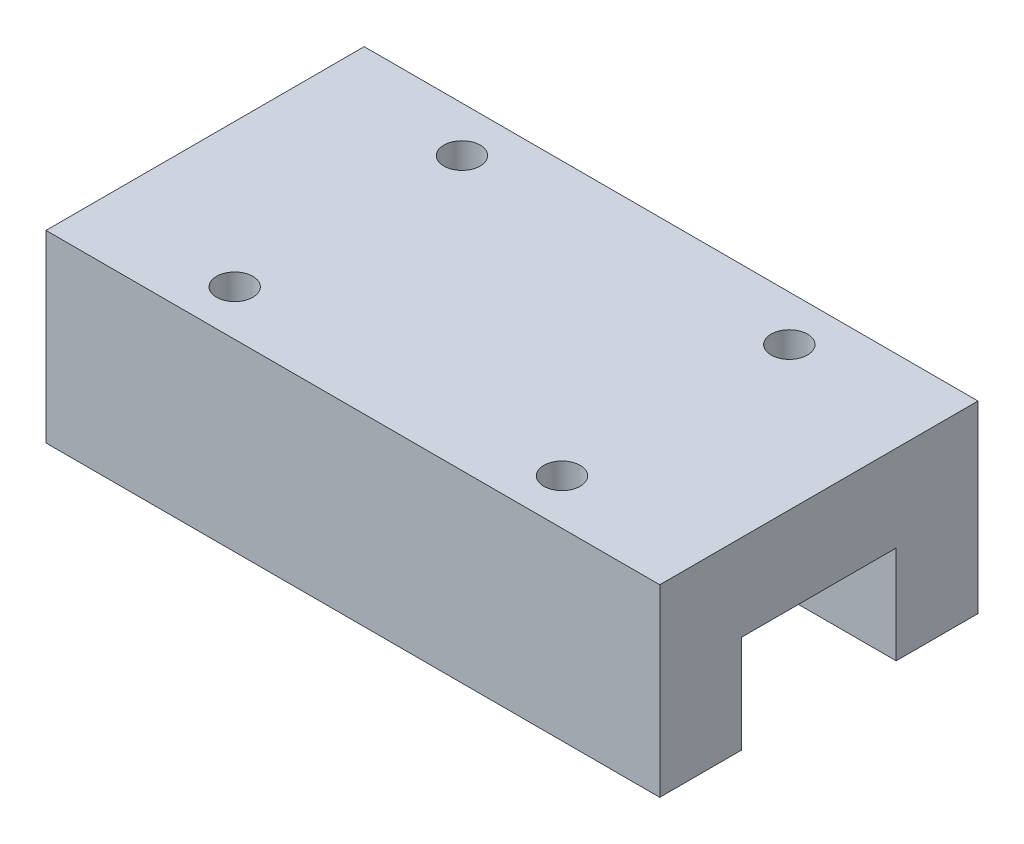
SolidWorks part; units mm, degrees
ref_plane "前视基准面" through (0, 0, 0) normal (0, 0, 1) x (1, 0, 0)
ref_plane "上视基准面" through (0, 0, 0) normal (0, 1, 0) x (1, 0, 0)
ref_plane "右视基准面" through (0, 0, 0) normal (1, 0, 0) x (0, 0, -1)
sketch "草图1" plane through (0, 0, 0) normal (0, 1, 0) x (1, 0, 0)
  line L1 (0, 0) -> (135, 0)
  line L2 (0, 0) -> (0, 70)
  line L3 (0, 70) -> (135, 70)
  line L4 (135, 0) -> (135, 70)
  dimension "D1" = 135
  dimension "D2" = 70
extrude "拉伸1" add sketch "草图1" along normal blind 40.5
sketch "草图2" plane through (0, 0, 0) normal (0, -1, 0) x (1, 0, 0)
  line L0 (135, 0) -> (135, -70) construction
  line L1 (135, -18) -> (0, -18)
  line L2 (135, -18) -> (135, -52)
  line L3 (135, -52) -> (0, -52)
  line L4 (0, -18) -> (0, -52)
  line L5 (0, -70) -> (0, 0) construction
  dimension "D1" = 34
  dimension "D2" = 18
extrude "切除-拉伸1" cut sketch "草图2" against normal blind 21.5
sketch "草图3" plane through (0, 40.5, 0) normal (0, 1, 0) x (-1, 0, 0)
  line L0 (0, 0) -> (-135, 0) construction
  line L1 (-135, 0) -> (-135, -70) construction
  circle A0 centre (-103.5, -60) radius 4
  circle A1 centre (-103.5, -10) radius 4
  circle A2 centre (-31.5, -60) radius 4
  circle A3 centre (-31.5, -10) radius 4
  dimension "D1" = 50
  dimension "D8" = 31.5
  dimension "D2" = 72
  dimension "D3" = 50
  dimension "D4" = 10
  dimension "D5" = 31.5
  dimension "D6" = 72
  dimension "D7" = 10
extrude "切除-拉伸2" cut sketch "草图3" against normal blind 16
